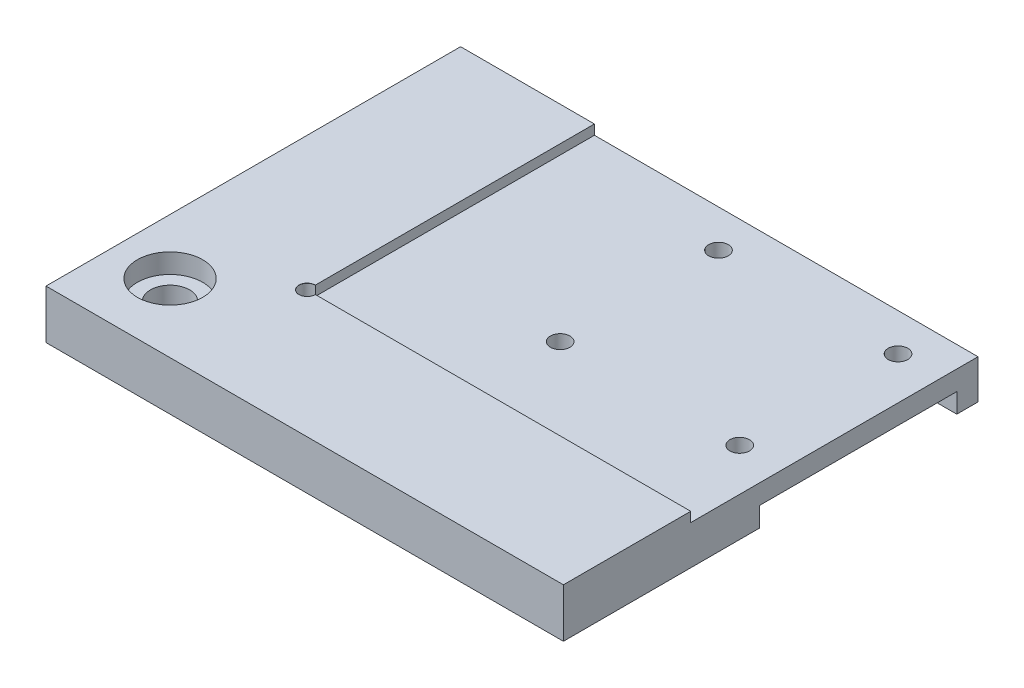
from build123d import *

# Parameters (mm, degrees)
SKETCH1_W                              = 158.5
SKETCH1_H                              = 127
BOSS_EXTRUDE1_DEPTH                    = 15
SKETCH2_W                              = 117.5
SKETCH2_H                              = 88
CUT_EXTRUDE1_DEPTH                     = 3
SKETCH3_W                              = 81
SKETCH3_H                              = 60.5
CUT_EXTRUDE2_DEPTH                     = 6
SKETCH4_W                              = 7
SKETCH4_H                              = 6
CUT_EXTRUDE3_DEPTH                     = 103.653847955
SKETCH5_R                              = 3
CUT_EXTRUDE4_DEPTH                     = 103.653847955
SKETCH6_R                              = 10
CUT_EXTRUDE5_DEPTH                     = 6
SKETCH7_R                              = 6
CUT_EXTRUDE6_DEPTH                     = 102.950049044
F_5_0MM_BLIND_DOWEL_HOLE_1_D           = 5
F_5_0MM_BLIND_DOWEL_HOLE_1_DEPTH       = 4
F_5_0MM_BLIND_DOWEL_HOLE_1_CSINK_D     = 5.05
F_5_0MM_BLIND_DOWEL_HOLE_1_CSINK_ANGLE = 90
F_5_0MM_BLIND_DOWEL_HOLE_1_TIP         = 1.502151548


with BuildPart() as part:
    # Sketch1 → Boss-Extrude1 (new body)
    with BuildSketch(Plane(origin=(0, 0, 0), x_dir=(1, 0, 0), z_dir=(0, 1, 0))):
        Rectangle(SKETCH1_W, SKETCH1_H)
    extrude(amount=BOSS_EXTRUDE1_DEPTH)

    # Sketch2 → Cut-Extrude1 (cut)
    with BuildSketch(Plane(origin=(0, 15, 0), x_dir=(1, 0, 0), z_dir=(0, 1, 0))):
        with Locations((20.5, 19.5)):
            Rectangle(SKETCH2_W, SKETCH2_H)
    extrude(amount=-CUT_EXTRUDE1_DEPTH, mode=Mode.SUBTRACT)

    # Sketch3 → Cut-Extrude2 (cut)
    with BuildSketch(Plane.XZ):
        with Locations((38.75, -26.75)):
            Rectangle(SKETCH3_W, SKETCH3_H)
    extrude(amount=-CUT_EXTRUDE2_DEPTH, mode=Mode.SUBTRACT)

    # Sketch4 → Cut-Extrude3 (cut, through all)
    with BuildSketch(Plane.XY):
        with Locations((1.75, 3)):
            Rectangle(SKETCH4_W, SKETCH4_H)
    extrude(amount=-CUT_EXTRUDE3_DEPTH, mode=Mode.SUBTRACT)

    # Sketch5 → Cut-Extrude4 (cut, through all)
    with BuildSketch(Plane(origin=(0, 15, 0), x_dir=(1, 0, 0), z_dir=(0, 1, 0))):
        with Locations(Location((11.25, 52, 0), (0, 0, 90))):
            Circle(SKETCH5_R)
        with Locations(Location((66.25, 52, 0), (0, 0, 90))):
            Circle(SKETCH5_R)
        with Locations(Location((66.25, 3.5, 0), (0, 0, 90))):
            Circle(SKETCH5_R)
        with Locations(Location((11.25, 3.5, 0), (0, 0, 90))):
            Circle(SKETCH5_R)
    extrude(amount=-CUT_EXTRUDE4_DEPTH, mode=Mode.SUBTRACT)

    # Sketch6 → Cut-Extrude5 (cut)
    with BuildSketch(Plane(origin=(0, 15, 0), x_dir=(1, 0, 0), z_dir=(0, 1, 0))):
        with Locations(Location((-62.25, -42.5, 0), (0, 0, 270))):
            Circle(SKETCH6_R)
    extrude(amount=-CUT_EXTRUDE5_DEPTH, mode=Mode.SUBTRACT)

    # Sketch7 → Cut-Extrude6 (cut, through all)
    with BuildSketch(Plane(origin=(0, 9, 0), x_dir=(1, 0, 0), z_dir=(0, 1, 0))):
        with Locations(Location((-62.25, -42.5, 0), (0, 0, 270))):
            Circle(SKETCH7_R)
    extrude(amount=-CUT_EXTRUDE6_DEPTH, mode=Mode.SUBTRACT)

    # Ø5.0mm blind dowel hole 1
    with Locations(Plane(origin=(0, 15, 0), x_dir=(1, 0, 0), z_dir=(0, 1, 0))):
        with Locations((-38.25, -24.5)):
            CounterSinkHole(F_5_0MM_BLIND_DOWEL_HOLE_1_D / 2, F_5_0MM_BLIND_DOWEL_HOLE_1_CSINK_D / 2, depth=F_5_0MM_BLIND_DOWEL_HOLE_1_DEPTH, counter_sink_angle=F_5_0MM_BLIND_DOWEL_HOLE_1_CSINK_ANGLE)
            with Locations((0, 0, -(F_5_0MM_BLIND_DOWEL_HOLE_1_DEPTH + F_5_0MM_BLIND_DOWEL_HOLE_1_TIP / 2))):  # 118° drill point
                Cone(0, F_5_0MM_BLIND_DOWEL_HOLE_1_D / 2, F_5_0MM_BLIND_DOWEL_HOLE_1_TIP, mode=Mode.SUBTRACT)


solid = part.part
